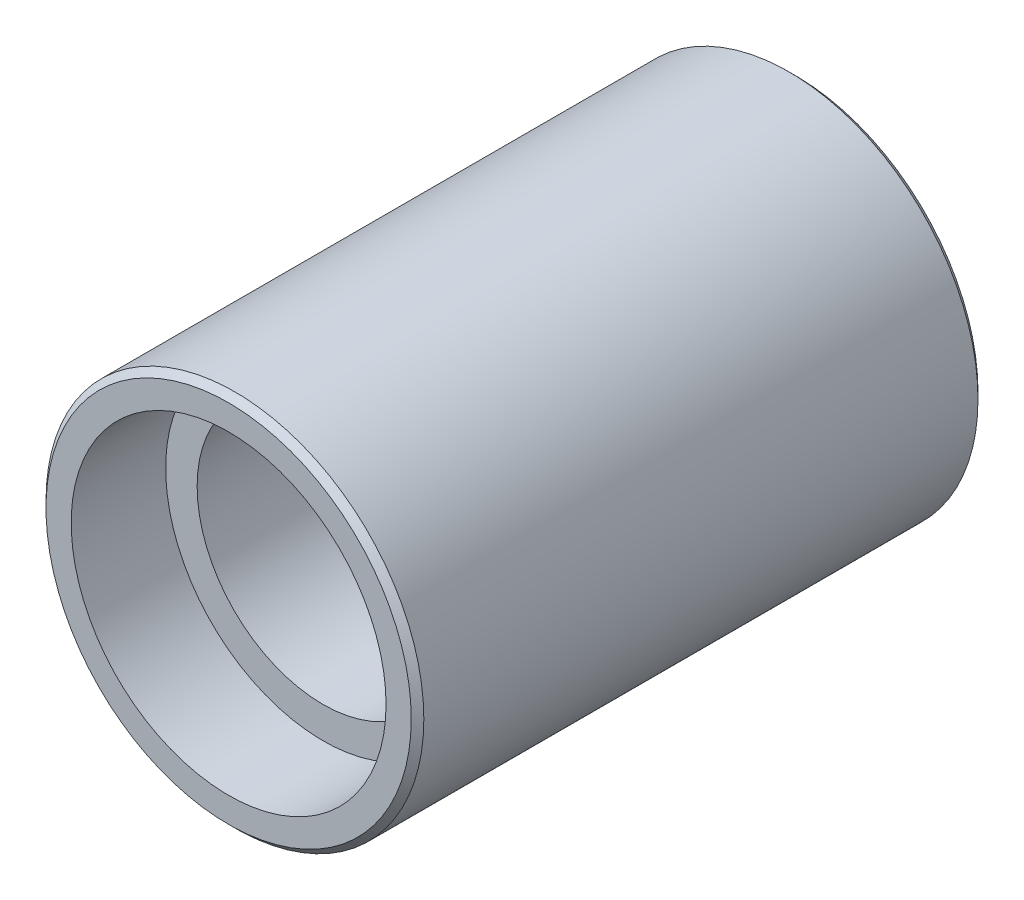
SolidWorks part; units mm, degrees
ref_plane "Front Plane" through (0, 0, 0) normal (0, 0, 1) x (1, 0, 0)
ref_plane "Top Plane" through (0, 0, 0) normal (0, 1, 0) x (1, 0, 0)
ref_plane "Right Plane" through (0, 0, 0) normal (1, 0, 0) x (0, 0, -1)
sketch "Sketch1" plane through (0, 0, 0) normal (0, 0, 1) x (1, 0, 0)
  circle A0 centre (0, 0) radius 6
  circle A1 centre (0, 0) radius 4
  dimension "D1" = 8
  dimension "D2" = 12
extrude "Boss-Extrude1" add sketch "Sketch1" along normal mid plane 18
sketch "Sketch2" plane through (0, 0, 9) normal (0, 0, 1) x (1, 0, 0)
  circle A0 centre (0, 0) radius 5
  dimension "D1" = 10
extrude "Cut-Extrude1" cut sketch "Sketch2" against normal blind 3
mirror "Mirror1" about plane through (0, 0, 0) normal (0, 0, 1) of "Cut-Extrude1"
chamfer "Chamfer1" distance 0.2 angle 45 2 edges at (6, 0, -9) (6, 0, 9)
